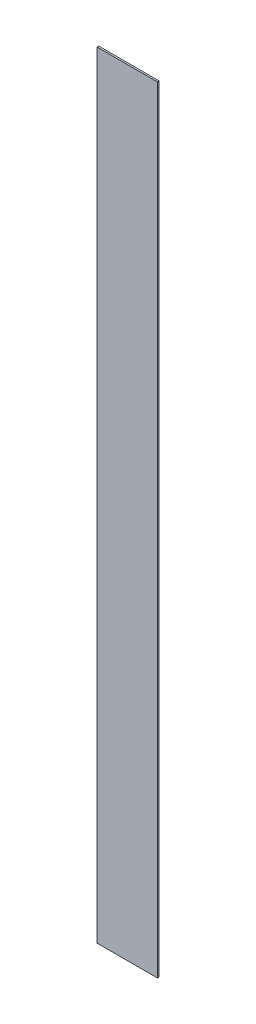
SolidWorks part; units mm, degrees
material "PMMA(有机玻璃)"
ref_plane "前视" through (0, 0, 0) normal (0, 0, 1) x (1, 0, 0)
ref_plane "上视" through (0, 0, 0) normal (0, 1, 0) x (1, 0, 0)
ref_plane "右视" through (0, 0, 0) normal (1, 0, 0) x (0, 0, -1)
sketch "草图1" plane through (0, 0, 0) normal (0, 0, 1) x (1, 0, 0)
  line L1 (-90, 1155) -> (90, 1155)
  line L2 (-90, 1155) -> (-90, -1155)
  line L3 (-90, -1155) -> (90, -1155)
  line L4 (90, 1155) -> (90, -1155)
  line L5 (-90, 1155) -> (90, -1155) construction
  line L6 (-90, -1155) -> (90, 1155) construction
  point P0 (0, 0)
  dimension "D1" = 2310
  dimension "D2" = 180
extrude "凸台-拉伸1" add sketch "草图1" along normal blind 5
hole_wizard "M5 间隙孔1" positions "草图3" profile "草图2" hole size "M5" standard "GB"
sketch "草图3" plane through (0, 0, 5) normal (0, 0, 1) x (1, 0, 0)
  line L0 (-427.5, 273) -> (-427.5, -273) construction
  line L1 (-427.5, -273) -> (427.5, -273) construction
  line L2 (0, 273) -> (0, -273) construction
  line L3 (427.5, 273) -> (-427.5, 273) construction
  line L5 (-427.5, 0) -> (427.5, 0) construction
  line L6 (427.5, -273) -> (427.5, 273) construction
  point P0 (-375, -261)
  point P46 (415.5, 250)
  point P48 (-415.5, 250)
  point P58 (-125, -261)
  point P59 (125, -261)
  point P61 (-125, 261)
  point P62 (125, 261)
  point P64 (-375, 261)
  point P88 (375, -261)
  point P89 (375, 261)
  point P108 (415.5, 0)
  point P109 (-415.5, 0)
  point P110 (415.5, -250)
  point P111 (-415.5, -250)
  dimension "D1" = 12
  dimension "D2" = 12
  dimension "D5" = 3
  dimension "D3" = 12
  dimension "D6" = 4
  dimension "D4" = 2
sketch "草图2" plane through (-375, -261, 5) normal (1, 0, 0) x (0, -1, 0)
  line L0 (0, 0) -> (0, 5)
  line L1 (0, 5) -> (2.75, 5)
  line L2 (2.75, 5) -> (2.75, 0)
  line L5 (2.75, 0) -> (0, 0)
  line L11 (0, -6.35) -> (0, 107.95) construction
  dimension "通孔孔直径" = 5.5
  dimension "通孔孔深度" = 5
